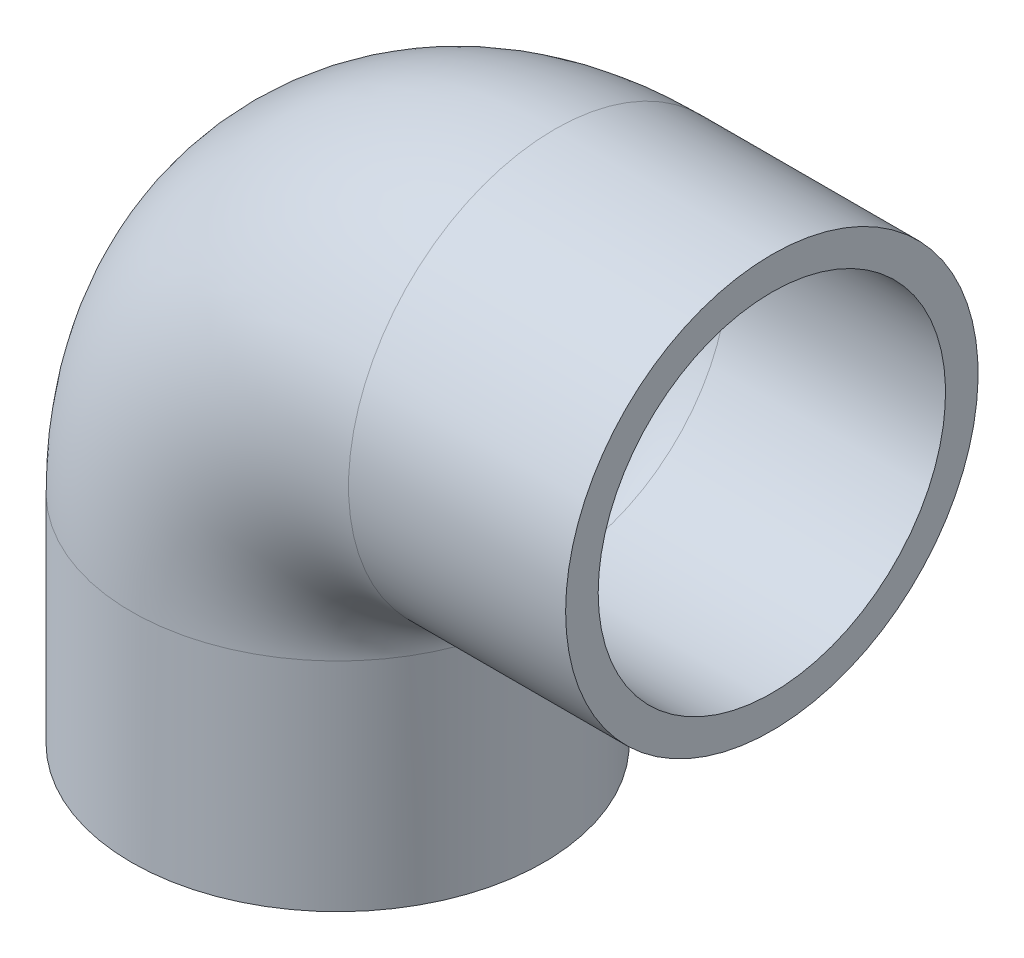
from build123d import *

# Parameters (mm, degrees)
SKETCH_2_R   = 19
SKETCH_2_R_2 = 16


with BuildPart() as part:
    # 扫描1: sweep along a path in 草图1
    with BuildLine(Plane.XY) as sweep_1_path:
        Line((0, 0), (0, 20))
        ThreePointArc((0, 20), (5.857864376, 34.142135624), (20, 40))
        Line((20, 40), (40, 40))
    # 草图2 → 扫描1 (sweep)
    with BuildSketch(Plane(origin=(0, 0, 0), x_dir=(1, 0, 0), z_dir=(0, 1, 0))):
        Circle(SKETCH_2_R)
        Circle(SKETCH_2_R_2, mode=Mode.SUBTRACT)
    sweep(path=sweep_1_path.line)


solid = part.part
